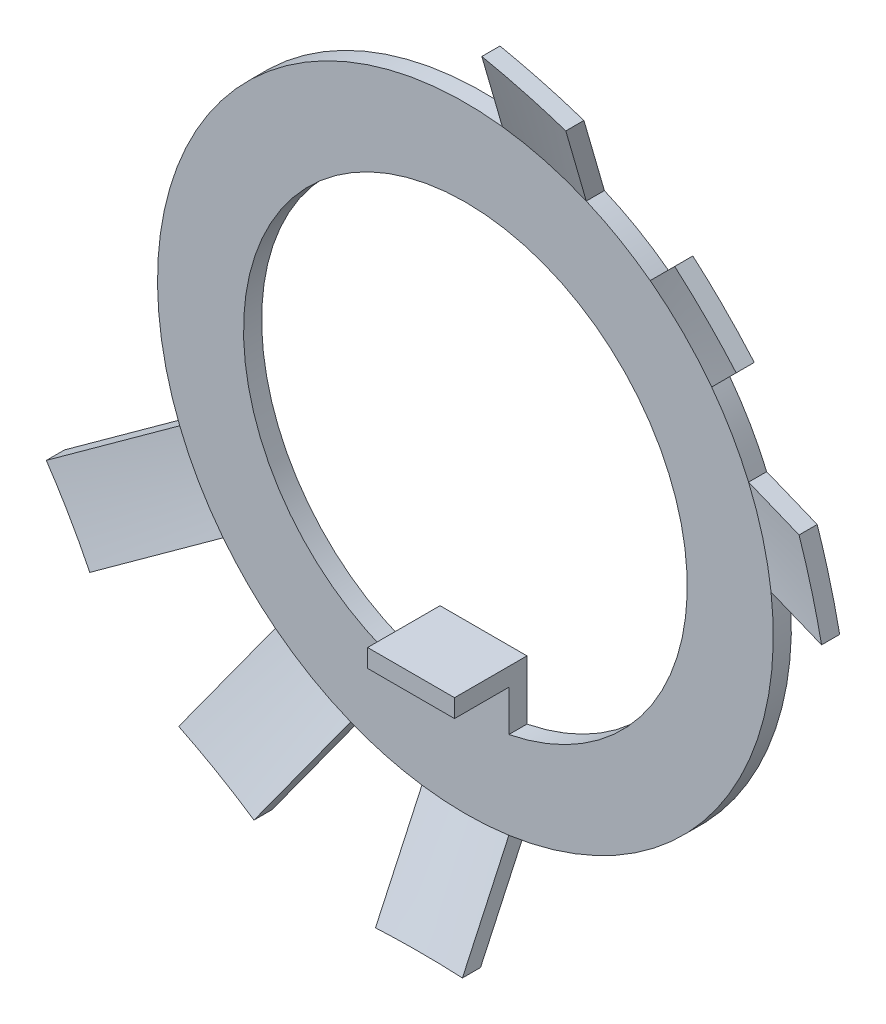
from build123d import *

# Parameters (mm, degrees)
CUT_EXTRUDE2_START  = -3e-06
SKETCH3_OUTSIDE_W   = 59.748
SKETCH3_OUTSIDE_H   = 59.748
CUT_EXTRUDE2_DEPTH  = 3.564697
SKETCH4_W           = 4.8
SKETCH4_H           = 1
BOSS_EXTRUDE1_DEPTH = 4


with BuildPart() as part:
    # Sketch2 → Boss-Revolve1 (revolve)
    with BuildSketch(Plane(origin=(0, 0, 0), x_dir=(0, 0, -1), z_dir=(1, 0, 0))):
        Polygon((-2.56469212, 22.5), (0, 17), (0, 0), (-1, 0), (-1, 17), (-3.56469212, 22.5), align=None)
    revolve(axis=Axis((0, 0, 0), (0, 0, 1)))

    # Sketch3 outside → Cut-Extrude2 (cut)
    # profile 1 of 2: a face of its own
    with BuildSketch(Plane.XY.offset(CUT_EXTRUDE2_START)):
        Rectangle(SKETCH3_OUTSIDE_W, SKETCH3_OUTSIDE_H)
        with BuildLine():
            Line((-2.4, -16.829735589), (-2.4, -22.371633825))
            Line((-2.4, -22.371633825), (2.4, -22.371633825))
            Line((2.4, -22.371633825), (2.4, -16.829735589))
            ThreePointArc((2.4, -16.829735589), (13.487006785, -10.348944293), (16.877441963, 2.037634111))
            Line((16.877441963, 2.037634111), (22.230504596, 3.471982921))
            Line((22.230504596, 3.471982921), (20.98817318, 8.108426887))
            Line((20.98817318, 8.108426887), (15.635110547, 6.674078078))
            ThreePointArc((15.635110547, 6.674078078), (14.722431864, 8.5), (13.597476435, 10.203363886))
            Line((13.597476435, 10.203363886), (17.516190259, 14.122077709))
            Line((17.516190259, 14.122077709), (14.122077709, 17.516190259))
            Line((14.122077709, 17.516190259), (10.203363886, 13.597476435))
            ThreePointArc((10.203363886, 13.597476435), (8.5, 14.722431864), (6.674078078, 15.635110547))
            Line((6.674078078, 15.635110547), (8.108426887, 20.98817318))
            Line((8.108426887, 20.98817318), (3.471982921, 22.230504596))
            Line((3.471982921, 22.230504596), (2.037634111, 16.877441963))
            ThreePointArc((2.037634111, 16.877441963), (-13.487006785, 10.348944293), (-15.774978559, -6.336406825))
            Line((-15.774978559, -6.336406825), (-20.574403217, -9.107355943))
            Line((-20.574403217, -9.107355943), (-18.174403217, -13.264277882))
            Line((-18.174403217, -13.264277882), (-13.374978559, -10.493328764))
            ThreePointArc((-13.374978559, -10.493328764), (-12.02081528, -12.02081528), (-10.493328764, -13.374978559))
            Line((-10.493328764, -13.374978559), (-13.264277882, -18.174403217))
            Line((-13.264277882, -18.174403217), (-9.107355943, -20.574403217))
            Line((-9.107355943, -20.574403217), (-6.336406825, -15.774978559))
            ThreePointArc((-6.336406825, -15.774978559), (-4.399923767, -16.420739047), (-2.4, -16.829735589))
        make_face(mode=Mode.SUBTRACT)
    # profile 2 of 2: a face of its own
    with BuildSketch(Plane.XY.offset(CUT_EXTRUDE2_START)):
        with BuildLine():
            Line((2.4, -12.012597554), (2.4, -8.75))
            Line((2.4, -8.75), (-2.4, -8.75))
            Line((-2.4, -8.75), (-2.4, -12.012597554))
            ThreePointArc((-2.4, -12.012597554), (0, 12.25), (2.4, -12.012597554))
        make_face()
    extrude(amount=CUT_EXTRUDE2_DEPTH, mode=Mode.SUBTRACT)

    # Sketch4 → Boss-Extrude1 (add)
    with BuildSketch(Plane.XY):
        with Locations((0, -9.25)):
            Rectangle(SKETCH4_W, SKETCH4_H)
    extrude(amount=BOSS_EXTRUDE1_DEPTH)


solid = part.part
